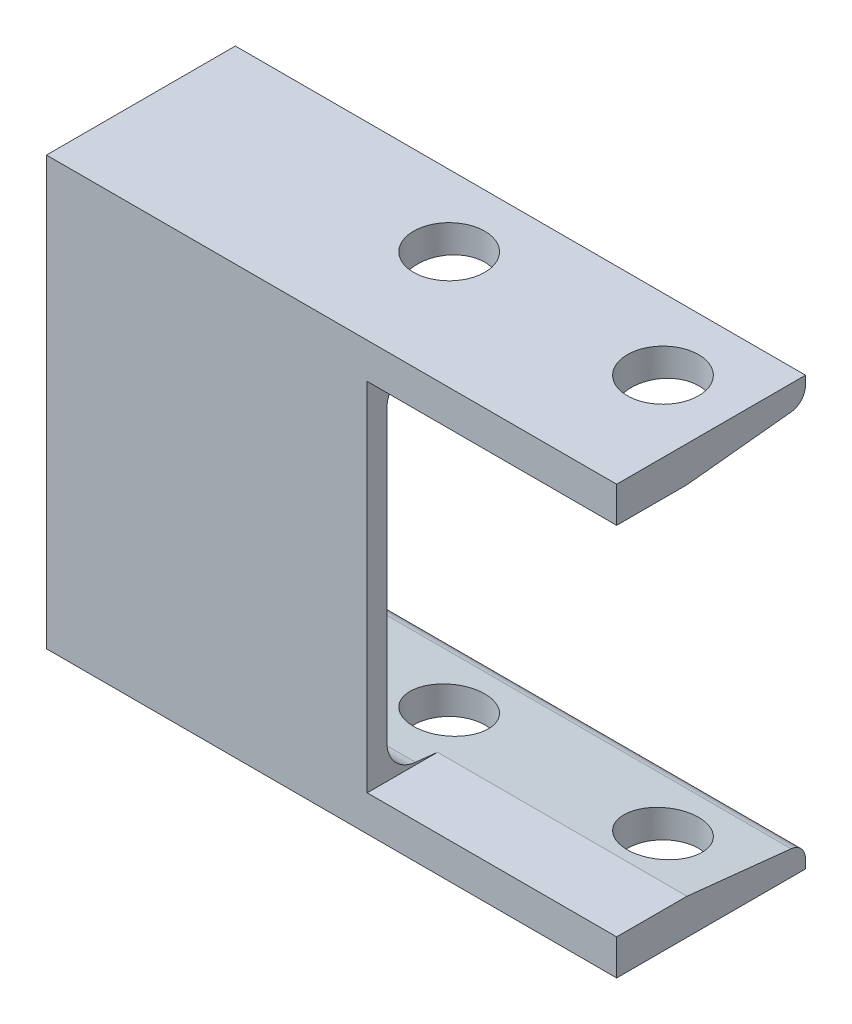
from build123d import *

# Parameters (mm, degrees)
C_CHANNEL_12_1_DEPTH = 160
SKETCH2_W            = 100
SKETCH2_H            = 100
CUT_EXTRUDE1_DEPTH   = 40
CUT_EXTRUDE2_REACH   = 208.903
SKETCH3_R            = 10


with BuildPart() as part:
    # Sketch11 → C-channel 12(1) (new body)
    with BuildSketch(Plane(origin=(0, 0, 0), x_dir=(0, 0, -1), z_dir=(1, 0, 0))):
        with BuildLine():
            Line((53, 120), (0, 120))
            Line((0, 120), (0, 0))
            Line((0, 0), (53, 0))
            Line((53, 0), (53, 2.451956213))
            ThreePointArc((53, 2.451956213), (51.844151715, 5.463043942), (48.970378085, 6.927304742))
            Line((48.970378085, 6.927304742), (13.559243831, 10.649164928))
            ThreePointArc((13.559243831, 10.649164928), (7.811696571, 13.577686529), (5.5, 19.599861986))
            Line((5.5, 19.599861986), (5.5, 100.400138014))
            ThreePointArc((5.5, 100.400138014), (7.811696571, 106.422313471), (13.559243831, 109.350835072))
            Line((13.559243831, 109.350835072), (48.970378085, 113.072695258))
            ThreePointArc((48.970378085, 113.072695258), (51.844151715, 114.536956058), (53, 117.548043787))
            Line((53, 117.548043787), (53, 120))
        make_face()
    extrude(amount=C_CHANNEL_12_1_DEPTH)

    # Sketch2 → Cut-Extrude1 (cut)
    with BuildSketch(Plane.XY):
        with Locations((140, 60)):
            Rectangle(SKETCH2_W, SKETCH2_H)
    extrude(amount=-CUT_EXTRUDE1_DEPTH, mode=Mode.SUBTRACT)

    # Cut-Extrude2: up to this face of the body (flat: up to its plane)
    cut_extrude2_end = Plane(part.part.faces().sort_by_distance((80, 120, -26.5))[0])
    # Sketch3 → Cut-Extrude2 (cut, up to the picked face)
    with BuildSketch(Plane.XZ, mode=Mode.PRIVATE) as cut_extrude2_sk1:
        with Locations(Location((140, -33, 0), (0, 0, 270))):
            Circle(SKETCH3_R)
    cut_extrude2_tool1 = split(extrude(cut_extrude2_sk1.sketch, amount=-CUT_EXTRUDE2_REACH, mode=Mode.PRIVATE), bisect_by=cut_extrude2_end, keep=Keep.BOTH, mode=Mode.PRIVATE)
    # Sketch3 → Cut-Extrude2 (cut, up to the picked face)
    with BuildSketch(Plane.XZ, mode=Mode.PRIVATE) as cut_extrude2_sk2:
        with Locations(Location((80, -33, 0), (0, 0, 270))):
            Circle(SKETCH3_R)
    cut_extrude2_tool2 = split(extrude(cut_extrude2_sk2.sketch, amount=-CUT_EXTRUDE2_REACH, mode=Mode.PRIVATE), bisect_by=cut_extrude2_end, keep=Keep.BOTH, mode=Mode.PRIVATE)
    add(cut_extrude2_tool1.solids().sort_by(Axis((140, 0, -33), (0, 1, 0)))[0], mode=Mode.SUBTRACT)
    add(cut_extrude2_tool2.solids().sort_by(Axis((80, 0, -33), (0, 1, 0)))[0], mode=Mode.SUBTRACT)


solid = part.part
